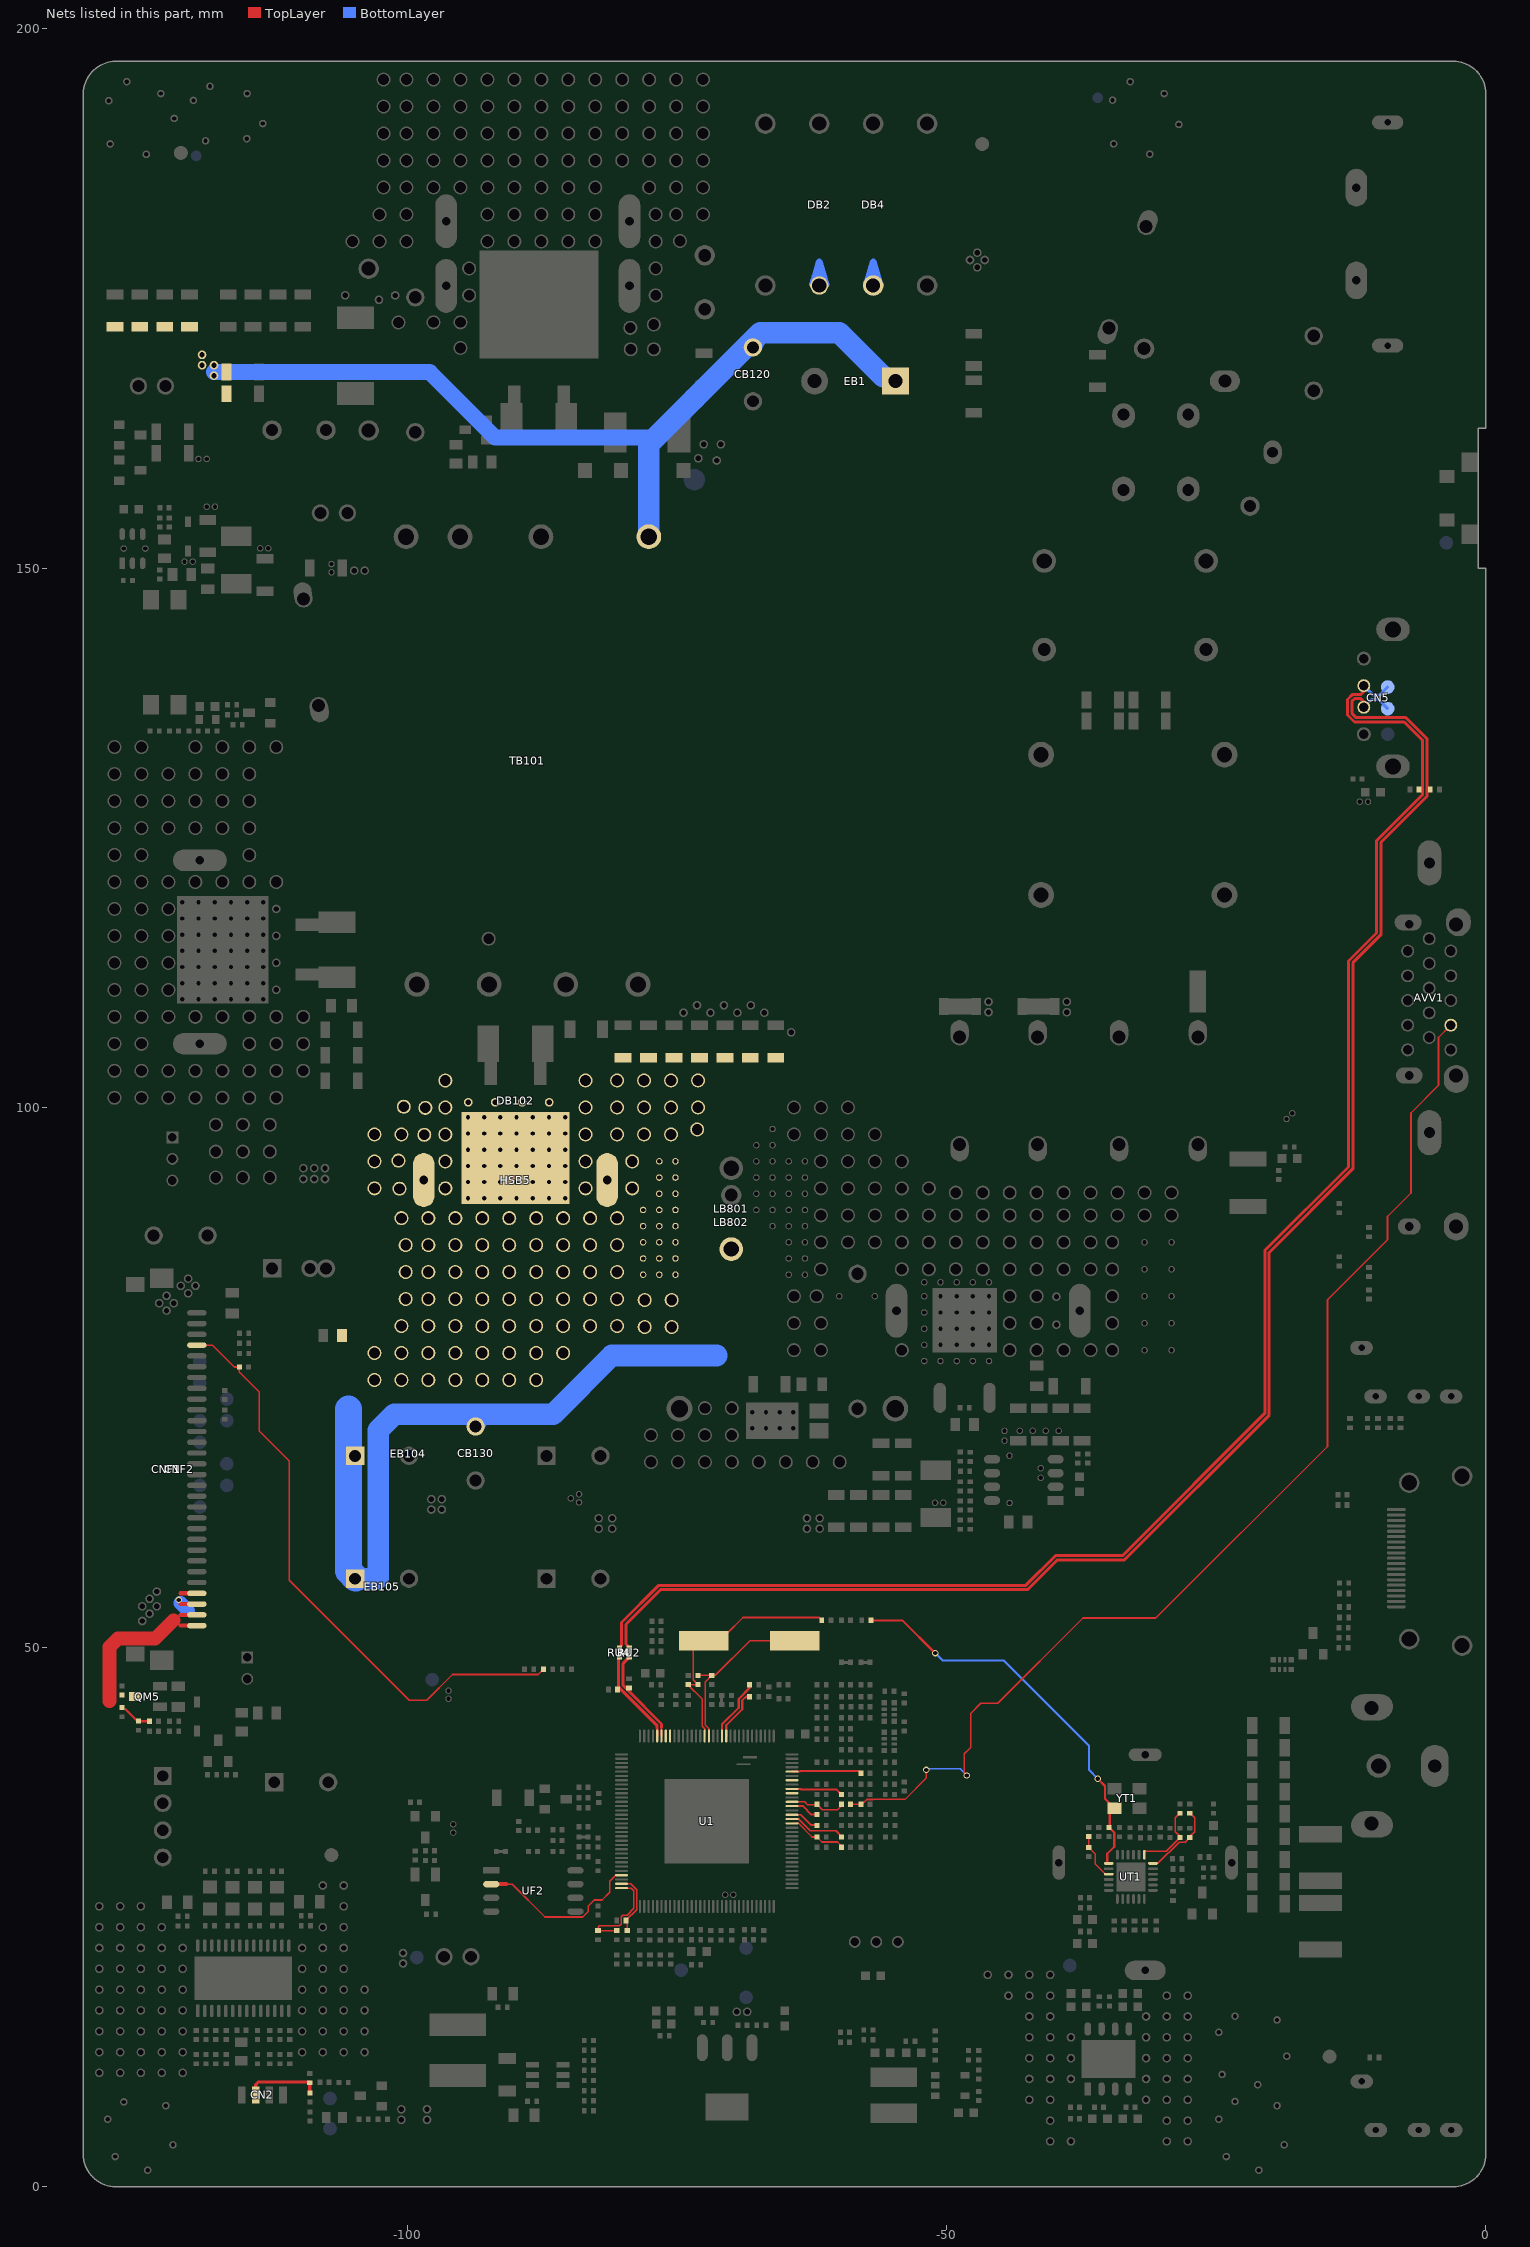
[diagram p0: the nets of this part, all layers, seen from the top]
# Altium PCB MISC84438.PcbDoc (part 13 of 15)
Units mm, origin at the board's own origin, x right, y up, seen from the top; angles counter-clockwise.
Board outline 130 x 197 mm, 2 copper layers (TopLayer, BottomLayer), stack 1.571 mm thick; 574 components, 314 nets, 2636 pads, 811 vias.

## Via types
v1: diameter 0.6, hole 0.4, TopLayer to BottomLayer, tented both sides, 780 vias
v2: diameter 0.7, hole 0.5, TopLayer to BottomLayer, tented both sides, 15 vias
v3: diameter 0.8, hole 0.6, TopLayer to BottomLayer, tented both sides, 12 vias
v4: diameter 0.8, hole 0.5, TopLayer to BottomLayer, tented both sides, 4 vias

## Nets (pads, with @x,y where several pads share a name; then routed paths per layer and width w, separated by ;. In a path a pad name is that pad's centre, name@x,y a point inside that pad or via, vN(x,y) a via of type N, cw(c..) or ccw(c..) an arc to the next point about the centre after c; other vN are vias at no path point) (continued)
SPI_DO: U1.93 UF2.2 | length 15.8
  TopLayer w0.152: -90.805,28.042 -90.246,28.042 -87.203,24.998 -83.721,24.998 -83.185,25.534 -83.185,26.035 -82.652,26.568 -81.928,26.568 -81.204,27.292 -81.204,28.308 -80.642,28.871 U1.93@-80.112,28.871
  TopLayer w0.381: UF2.2@-92.19,28.042 -90.805,28.042
T-IF-AGC: CT1.2 RT2.1 UT1.15 | length 4.4
  TopLayer w0.152: RT2.1@-36.804,32.455 CT1.2@-36.805,31.438 -36.22,30.854 -36.22,29.938 -35.247,28.964 UT1.15@-34.956,28.964
TUNER_SCL: CT8.2 RT6.2 UT1.6 | length 7
  TopLayer w0.127: UT1.6@-30.856,29.964 -30.389,29.964 -28.426,31.928 -27.871,31.928 CT8.2@-27.432,32.366 -27.432,32.472 -26.991,32.912 -26.991,34.174 RT6.2@-27.432,34.614
TUNER_SDA: CT7.2 RT5.2 UT1.7 | length 6.7
  TopLayer w0.127: UT1.7@-31.656,30.764 -31.656,31.019 -31.585,31.09 -29.623,31.09 CT7.2@-28.346,32.366 -28.346,32.472 -28.787,32.912 -28.787,34.174 RT5.2@-28.347,34.614
UART_RX: DH9.K RF11.2 U1.96 | length 9.4
  TopLayer w0.127: RF11.2@-80.543,23.739 DH9.K@-82.296,23.739 -82.296,24.041 -82.169,24.168 -80.313,24.168 -80.146,24.335 -80.146,25.024 -80.016,25.154 -79.606,25.154 -78.969,25.791 -78.969,27.409 -79.231,27.671 U1.96@-80.112,27.671
UART_TX: DH8.K RF10.2 U1.95 | length 6.4
  TopLayer w0.127: U1.95@-80.654,28.071 U1.95@-80.112,28.071 -79.271,28.071 -78.715,27.514 -78.715,25.686 DH8.K@-79.712,24.689 -79.578,24.555 RF10.2@-79.578,23.739
USB0_DM: DU2.K RU2.2 RU2.3 U1.59 | length 9
  TopLayer w0.203: U1.59@-76.412,41.771 -76.412,42.545
  TopLayer w0.279: RU2.2@-79.39,49.079 -79.967,48.502 -79.967,46.453 -79.587,46.073 -76.406,42.892 -76.406,42.551
USB0_DP: DU1.K RU4.2 RU4.3 U1.60 | length 8.8
  TopLayer w0.203: U1.60@-76.812,41.771 -76.812,42.532
  TopLayer w0.279: RU4.2@-80.305,49.079 -80.374,49.01 -80.374,46.285 -80.332,46.243 -76.812,42.723 -76.812,42.532
USB0_M: CN5.2@-11.31,137.13 DU4.K RU2.1 USB0_M.1 | length 152.5
  TopLayer w0.279: RU2.1@-79.39,49.981 -79.705,50.296 -79.705,52.129 -76.5,55.334 -42.477,55.334 -39.708,58.102 -33.485,58.102 -20.079,71.509 -20.079,86.597 -12.332,94.344 -12.332,113.436 -9.728,116.039 -9.728,124.596 -5.448,128.876 -5.448,129.488 -5.448,134.217 -7.401,136.169 -12.014,136.169 -12.421,136.576 -12.421,137.677 -12.171,137.927 -11.587,137.927 -11.31,137.65 CN5.2@-11.31,137.13
  BottomLayer w0.279: CN5.2@-11.31,137.13 -10.594,137.846 -9.942,137.846 USB0_M.1@-9.096,137
USB0_P: CN5.3@-11.31,139.13 DU3.K RU4.1 USB0_P.1 | length 153.1
  TopLayer w0.279: RU4.1@-80.305,49.981 -80.112,50.174 -80.112,52.297 -76.669,55.74 -42.645,55.74 -39.877,58.509 -33.654,58.509 -20.485,71.677 -20.485,86.765 -12.738,94.512 -12.738,113.604 -10.135,116.207 -10.135,124.765 -5.855,129.045 -5.855,129.488 -5.855,134.048 -7.569,135.763 -12.183,135.763 -12.827,136.407 -12.827,137.846 -12.34,138.333 -11.578,138.333 -11.31,138.601 CN5.3@-11.31,139.13
  BottomLayer w0.279: CN5.3@-11.31,139.13 -10.432,138.252 -9.844,138.252 USB0_P.1@-9.096,139
USB1_DM: U1.57
USB1_DP: U1.58
VBL: CB130.2 DB102.2 EB104.1@-104.811,67.742 EB105.1@-104.811,56.35 HSB5.1@-81.448,93.305 HSB5.2 LB801.1@-69.945,86.9 LB802.1 pad.VIA5@-73.1,98 pad.VIA5@-73.023,100.036 pad.VIA5@-73.023,102.536 pad.VIA5@-75.115,84.535 pad.VIA5@-75.115,86.035 pad.VIA5@-75.115,87.535 pad.VIA5@-75.115,89.035 pad.VIA5@-75.115,90.535 pad.VIA5@-75.115,92.035 pad.VIA5@-75.115,93.535 pad.VIA5@-75.115,95.035 pad.VIA5@-75.467,79.68 pad.VIA5@-75.467,82.18 pad.VIA5@-75.523,97.536 pad.VIA5@-75.523,100.036 pad.VIA5@-75.523,102.536 pad.VIA5@-76.615,84.535 pad.VIA5@-76.615,86.035 pad.VIA5@-76.615,87.535 pad.VIA5@-76.615,89.035 pad.VIA5@-76.615,90.535 pad.VIA5@-76.615,92.035 pad.VIA5@-76.615,93.535 pad.VIA5@-76.615,95.035 pad.VIA5@-77.967,79.68 pad.VIA5@-77.967,82.18 pad.VIA5@-78.023,97.536 pad.VIA5@-78.023,100.036 pad.VIA5@-78.023,102.536 pad.VIA5@-78.115,84.535 pad.VIA5@-78.115,86.035 pad.VIA5@-78.115,87.535 pad.VIA5@-78.115,89.035 pad.VIA5@-78.115,90.535 pad.VIA5@-79.123,92.536 pad.VIA5@-79.123,95.036 pad.VIA5@-80.523,79.771 pad.VIA5@-80.523,82.271 pad.VIA5@-80.523,84.771 pad.VIA5@-80.523,87.271 pad.VIA5@-80.523,89.771 pad.VIA5@-80.523,97.536 pad.VIA5@-80.523,100.036 pad.VIA5@-80.523,102.536 pad.VIA5@-83.023,79.771 pad.VIA5@-83.023,82.271 pad.VIA5@-83.023,84.771 pad.VIA5@-83.023,87.271 pad.VIA5@-83.023,89.771 pad.VIA5@-83.448,92.536 pad.VIA5@-83.448,95.036 pad.VIA5@-83.448,97.536 pad.VIA5@-83.448,100.036 pad.VIA5@-83.448,102.536 pad.VIA5@-85.343,91.615 pad.VIA5@-85.343,93.115 pad.VIA5@-85.343,94.615 pad.VIA5@-85.343,96.115 pad.VIA5@-85.343,97.615 pad.VIA5@-85.343,99.115 pad.VIA5@-85.523,77.271 pad.VIA5@-85.523,79.771 pad.VIA5@-85.523,82.271 pad.VIA5@-85.523,84.771 pad.VIA5@-85.523,87.271 pad.VIA5@-85.523,89.771 pad.VIA5@-86.823,100.508 pad.VIA5@-86.843,91.615 pad.VIA5@-86.843,93.115 pad.VIA5@-86.843,94.615 pad.VIA5@-86.843,96.115 pad.VIA5@-86.843,97.615 pad.VIA5@-86.843,99.115 pad.VIA5@-88.023,74.771 pad.VIA5@-88.023,77.271 pad.VIA5@-88.023,79.771 pad.VIA5@-88.023,82.271 pad.VIA5@-88.023,84.771 pad.VIA5@-88.023,87.271 pad.VIA5@-88.023,89.771 pad.VIA5@-88.343,91.615 pad.VIA5@-88.343,93.115 pad.VIA5@-88.343,94.615 pad.VIA5@-88.343,96.115 pad.VIA5@-88.343,97.615 pad.VIA5@-88.343,99.115 pad.VIA5@-89.323,100.508 pad.VIA5@-89.843,91.615 pad.VIA5@-89.843,93.115 pad.VIA5@-89.843,94.615 pad.VIA5@-89.843,96.115 pad.VIA5@-89.843,97.615 pad.VIA5@-89.843,99.115 pad.VIA5@-90.523,74.771 pad.VIA5@-90.523,77.271 pad.VIA5@-90.523,79.771 pad.VIA5@-90.523,82.271 pad.VIA5@-90.523,84.771 pad.VIA5@-90.523,87.271 pad.VIA5@-90.523,89.771 pad.VIA5@-91.343,91.615 pad.VIA5@-91.343,93.115 pad.VIA5@-91.343,94.615 pad.VIA5@-91.343,96.115 pad.VIA5@-91.343,97.615 pad.VIA5@-91.343,99.115 pad.VIA5@-91.823,100.508 pad.VIA5@-92.843,91.615 pad.VIA5@-92.843,93.115 pad.VIA5@-92.843,94.615 pad.VIA5@-92.843,96.115 pad.VIA5@-92.843,97.615 pad.VIA5@-92.843,99.115 pad.VIA5@-93.023,74.771 pad.VIA5@-93.023,77.271 pad.VIA5@-93.023,79.771 pad.VIA5@-93.023,82.271 pad.VIA5@-93.023,84.771 pad.VIA5@-93.023,87.271 pad.VIA5@-93.023,89.771 pad.VIA5@-94.323,100.508 pad.VIA5@-94.343,91.615 pad.VIA5@-94.343,93.115 pad.VIA5@-94.343,94.615 pad.VIA5@-94.343,96.115 pad.VIA5@-94.343,97.615 pad.VIA5@-94.343,99.115 pad.VIA5@-95.523,74.771 pad.VIA5@-95.523,77.271 pad.VIA5@-95.523,79.771 pad.VIA5@-95.523,82.271 pad.VIA5@-95.523,84.771 pad.VIA5@-95.523,87.271 pad.VIA5@-95.523,89.771 pad.VIA5@-96.447,92.536 pad.VIA5@-96.447,95.036 pad.VIA5@-96.447,97.527 pad.VIA5@-96.447,100.027 pad.VIA5@-96.447,102.527 pad.VIA5@-98.3,100 pad.VIA5@-98.4,97.5 pad.VIA5@-98.023,74.771 pad.VIA5@-98.023,77.271 pad.VIA5@-98.023,79.771 pad.VIA5@-98.023,82.271 pad.VIA5@-98.023,84.771 pad.VIA5@-98.023,87.271 pad.VIA5@-98.023,89.771 pad.VIA5@-100.3,100.1 pad.VIA5@-100.7,92.5 pad.VIA5@-100.8,95.1 pad.VIA5@-100.123,82.271 pad.VIA5@-100.123,84.771 pad.VIA5@-100.123,87.271 pad.VIA5@-100.523,74.771 pad.VIA5@-100.523,77.271 pad.VIA5@-100.523,79.771 pad.VIA5@-100.523,89.771 pad.VIA5@-100.523,97.536 pad.VIA5@-103.023,74.771 pad.VIA5@-103.023,77.271 pad.VIA5@-103.023,92.536 pad.VIA5@-103.023,95.036 pad.VIA5@-103.023,97.536 RB124.2 RB125.2 RB126.2 RB127.2 RB140.1 RB162.2 RB163.2 RB164.2 | length 66
  BottomLayer w2: EB105.1@-104.811,56.35 -102.743,56.35 -102.664,56.429 -102.664,70.107 -101.171,71.599 -92.745,71.599 -92.497,71.599 -92.341,71.599 -86.453,71.599 -81.014,77.038 -71.298,77.038
  BottomLayer w2.54: -105.42,72.08 -105.42,68.706 -105.42,68.351 -105.42,67.783 -105.42,57.314 -105.42,57.072 EB105.1@-104.762,56.413
Vbridge: CB120.2 DB2.K DB4.K EB1.1@-54.708,167.359 pad.VIA5@-117.892,167.875 pad.VIA5@-117.892,168.84 pad.VIA5@-118.999,168.834 pad.VIA5@-118.999,169.799 RB117.2 RB118.2 RB150.2 RB151.2 RB152.2 RB156.2 TB101.1 TP-TDT.1 | length 79.7
  BottomLayer w1.5: pad.VIA5@-117.892,168.199 -97.892,168.199 -91.821,162.128 -76.975,162.128
  BottomLayer w2: TB101.1@-77.585,152.942 -77.585,161.518 -76.975,162.128 -68.182,170.92 -67.272,171.831 -66.725,171.831 -66.597,171.831 -66.517,171.831 -59.931,171.831 EB1.1@-55.853,167.752
VCC_PANEL: CF38.1 CM4.1 CM7.2 CNF1.27 CNF1.28 CNF1.29 CNF1.30 CNF2.27 CNF2.28 CNF2.29 CNF2.30 QM5.D RM6.1 VCC_PANEL.1 | length 21.7
  TopLayer w0.203: -126.086,44.247 -124.999,43.16 RM6.1@-124.892,43.16 -124.873,43.142 CM7.2@-123.882,43.142
  TopLayer w0.381: -121.004,52 CNF2.30@-119.486,52 ; -121.004,53 CNF2.29@-119.486,53 ; -121.004,54 CNF2.28@-119.486,54 ; -121.004,55 CNF2.27@-119.486,55
  TopLayer w1.27: -127.584,44.983 -127.584,50.013 -126.785,50.812 -123.33,50.812 -121.641,52.502
  BottomLayer w1.27: -120.999,54.091 VCC_PANEL.1@-120.326,53.418
  other v1: -121.156,54.379
VCOM0: CF26.1 U1.28 | length 6.5
  TopLayer w0.198: U1.28@-64.312,38.471 -63.611,38.471 -63.546,38.536 -58.163,38.536 CF26.1@-57.931,38.303
VGA_BIN: CV7.1 U1.17 | length 5.3
  TopLayer w0.18: -63.692,34.071 -62.608,32.987 -60.234,32.987 CV7.1@-59.734,32.487
  TopLayer w0.198: U1.17@-64.312,34.071 -63.692,34.071 ; CV7.1@-59.734,32.41 CV7.1@-59.734,32.487
VGA_GIN: CV3.1 U1.18 | length 2.7
  TopLayer w0.18: U1.18@-64.312,34.471 -63.503,34.471 -62.56,33.528 CV3.1@-62.02,33.528
VGA_HS: CV9.2 RV12.2 U1.16 | length 5.5
  TopLayer w0.152: U1.16@-64.312,33.671 -63.719,33.671 -62.459,32.41 CV9.2@-61.995,32.41 -61.533,31.948 -60.092,31.948 RV12.2@-59.715,31.572
VGA_RIN: CV1.1 U1.20 | length 2.6
  TopLayer w0.18: U1.20@-64.312,35.271 -63.287,35.271 -62.509,34.493 CV1.1@-61.995,34.493
VGA_VS: CV10.2 RV10.2 U1.21 | length 5.2
  TopLayer w0.152: U1.21@-64.312,35.671 -63.144,35.671 -62.881,35.407 CV10.2@-61.995,35.407 ; CV10.2@-61.995,35.433 -61.508,34.946 -60.1,34.946 -59.734,35.313 RV10.2@-59.734,35.433
VIFM: CT23.2 U1.45 | length 5.8
  TopLayer w0.203: U1.45@-70.812,41.771 -70.812,42.832 -69.253,44.391 -69.253,45.21 -68.25,46.213 CT23.2@-68.25,46.507
VIFP: CT20.2 U1.44 | length 4.7
  TopLayer w0.203: U1.44@-70.412,41.771 -70.412,42.765 -68.923,44.254 -68.923,45.073 -68.581,45.415 CT20.2@-68.25,45.415
Vs: CK4.1 CN2.2 RK13.2 | length 7
  TopLayer w0.305: CN2.2@-114.035,8.502 -114.035,9.434 -113.767,9.703 CK4.1@-109.004,9.703 ; RK13.2@-109.004,8.705 CK4.1@-109.004,9.633
VS_VGA: AVV1.14 RV10.1 RV14.1 | length 106
  TopLayer w0.152: RV10.1@-58.884,35.433 RV14.1@-57.931,35.433 ; RV14.1@-57.931,35.44 RV14.1@-57.931,35.433 ; v1(-51.862,38.625) -51.862,37.87 -53.838,35.894 -56.771,35.894 -56.779,35.886 -57.39,35.886 -57.843,35.433 RV14.1@-57.931,35.433 ; v1(-48.112,38.111) -48.336,38.334 -48.336,40.119 -47.758,40.697 -47.758,43.851 -46.816,44.793 -45.246,44.793 -37.334,52.705 -30.587,52.705 -14.681,68.611 -14.681,80.772 -14.681,82.21 -9.119,87.772 -9.119,89.924 -6.934,92.109 -6.934,99.526 -4.383,102.078 -4.383,106.525 AVV1.14@-3.247,107.66
  BottomLayer w0.152: v1(-51.862,38.625) -51.765,38.722 -48.714,38.722 -48.112,38.12 v1(-48.112,38.111)
WP//SCL: CNF1.4 CNF2.4 RF22.2 RF25.2 | length 55.8
  TopLayer w0.152: CNF2.4@-119.486,78 -118.037,78 -116.009,75.972 RF22.2@-115.543,75.972 -115.543,75.506 -113.695,73.658 -113.695,70.047 -110.915,67.267 -110.915,56.2 -99.8,45.085 -98.168,45.085 -95.78,47.473 -87.826,47.473 RF25.2@-87.344,47.955
XTAL_O: CF40.1 CT14.2 UT1.13 YT1.1 | length 37.8
  TopLayer w0.203: CF40.1@-57.004,52.489 -54.089,52.489 -51.063,49.463 v1(-51.038,49.463) ; v1(-35.97,37.822) -35.294,37.146 -35.294,35.958 YT1.1@-34.415,35.079 ; UT1.13@-35.244,29.964 -35.1,30.109 ; UT1.13@-34.956,29.964 -35.1,30.109 ; YT1.1@-34.868,35.219 -34.868,33.361 CT14.2@-34.925,33.305 -34.446,32.826 -34.446,31.505 -35.1,30.851 -35.1,30.109
  BottomLayer w0.203: v1(-51.038,49.463) -50.343,48.768 -44.68,48.768 -36.788,40.876 -36.788,38.64 v1(-35.97,37.822)
XTALI: CF4.2 RF1.1 U1.48 YF1.1 | length 16.3
  TopLayer w0.152: RF1.1@-73.025,47.389 CF4.2@-71.755,47.389 ; U1.48@-72.012,41.771 -72.012,42.434 -72.365,42.786 -72.365,46.78 CF4.2@-71.755,47.389 ; YF1.1@-64.068,50.594 -68.215,50.594 -71.419,47.389 CF4.2@-71.755,47.389
XTALO: CF1.2 RF1.2 RF24.2 U1.49 YF1.2 | length 20.8
  TopLayer w0.152: RF1.2@-73.034,46.53 -73.965,46.53 -72.644,45.209 -72.644,42.671 -72.412,42.439 U1.49@-72.412,41.771 ; RF1.2@-73.025,46.539 -73.478,46.993 -73.478,49.988 -72.872,50.594 YF1.2@-72.483,50.594 ; YF1.2@-70.358,51.257 -68.859,52.756 -61.817,52.756 RF24.2@-61.55,52.489
YPBPR_PB: U1.23
YPBPR_PR: U1.26
YPBPR_Y: CI1.1 U1.24 | length 4.8
  TopLayer w0.198: U1.24@-64.312,36.871 -63.525,36.871
  TopLayer w0.203: -63.525,36.871 -63.48,36.826 -60.213,36.826 CI1.1@-59.734,36.347
pads on no net: "Conformal Coating.0" AI_V.0 AI_V.1 AI_V.2 AVH1.4@-2.9,50.55 AVH1.4@-2.9,65.45 AVH1.4@-7.2,50.75 AVH1.4@-7.2,65.25 AVI1.0 AVI2.0 AVO1.0 AVO2.0 AVO2.4 AVV1.0 AVV1.4 AVV1.9 AVV1.11 AVV1.30 AVV1.31 AVV1.32 AVV1.33 AVV1.34 AVV1.35 AVV1.36 AVV1.37 AVV1.38 AVV1.39 AVV1.40 AVV1.41 AVV1.42 AVV1.43 AVV1.44 BB101.35 BB101.36 BB801.35 BB801.36 CB114.1@-107.507,162.814 CB114.1@-112.507,162.814 CB116.0 CB120.41 CB120.42 CB130.41 CB130.42 CB808.41 CB808.42 CN5.0 CN5.1@-11.31,137.13 CN5.2@-11.31,139.13 CN5.3@-11.31,141.63 CN9.0 CNA1.0 CNA2.0 CNA3.0 CNB1.0 CNB1.1@-9.1,170.65 CNB1.1@-9.1,191.35 CNB1.1@-12,176.7 CNB1.1@-12,185.3 CNB1.3 CNB1.4 CNB2.0 CNB832.0 CNB833.0 CXB1.77 CXB1.78 CXB2.3 CXB2.4 CYB1.61 CYB2.61 CYB3.61 CYB4.61 CYB5.61 CYB6.61 DB1.15 DB1.16 DB2.15 DB2.16 DB3.15 DB3.16 DB4.15 DB4.16 DB106.15 DB106.16 DB801.0 DB801.1 EA1.0 EA1.1@-107.304,37.486 EA1.1@-112.304,37.486 EB1.1@-54.708,167.359 EB1.1@-62.208,167.359 EB101.0 EB101.1@-107.5,85.114 EB101.1@-112.5,85.114 EB102.1@-109,85.114 EB102.1@-112.5,85.114 EB104.0 EB104.1@-99.811,67.742 EB104.1@-104.811,67.742 EB105.0 EB105.1@-99.811,56.35 EB105.1@-104.811,56.35 EB106.0 EB107.0 EB801.0 EB801.1@-82.073,67.742 EB801.1@-87.073,67.742 EB802.0 EB802.1@-82.073,56.35 EB802.1@-87.073,56.35 ED2.0 ED2.5 ED2.6 FB1.4 FB1.5 H1.0 H1.1@-19.225,5.725 H1.1@-20.34,7.339 H1.1@-22.232,7.859 H1.1@-24.015,7.041 H1.1@-24.856,5.268 H2.0 H2.1@-19.225,13.725 H2.1@-19.408,11.772 H2.1@-20.34,15.339 H2.1@-20.804,10.393 H2.1@-22.76,10.234 H2.1@-22.232,15.859 H2.1@-24.015,15.041 H2.1@-24.36,11.37 H2.1@-24.856,13.268 H3.0 H3.1@-122.225,5.725 H3.1@-123.34,7.339 H3.1@-125.232,7.859 H3.1@-127.015,7.041 H3.1@-127.856,5.268 H4.0 H4.1@-29.225,192.725 H4.1@-29.408,190.772 H4.1@-30.804,189.393 H4.1@-32.76,189.234 H4.1@-34.36,190.37 H4.1@-34.856,192.268 H5.0 H5.1@-122.225,192.725 H5.1@-122.408,190.772 H5.1@-123.804,189.393 H5.1@-125.76,189.234 H5.1@-127.36,190.37 H5.1@-127.856,192.268 H6.0 H6.1@-114.225,192.725 H6.1@-114.408,190.772 H6.1@-115.804,189.393 H6.1@-117.76,189.234 H6.1@-119.36,190.37 H6.1@-119.856,192.268 HSB1.1@-79.374,176.188 HSB1.1@-96.374,176.188 HSB2.1@-79.374,182.188 HSB2.1@-96.374,182.188 HSB3.1@-119.2,105.938 HSB3.1@-119.2,122.938 HSB4.1@-37.626,81.193 HSB4.1@-54.626,81.193 HSB5.1@-81.448,93.305 HSB5.1@-98.448,93.305 JP1.1@-27.582,157.263 JP1.1@-27.582,164.263 JP2.1@-33.582,157.263 JP2.1@-33.582,164.263 LB801.1@-69.945,86.9 LB801.1@-69.946,94.4 LB802.3 LB802.4 LCB1.5 LCB1.6 LCB1.7 LCB1.8 LCB2.0 M1.0 M2.0 M3.0 M4.0 Manufacture_Info.0 MOVB1.2@-24.182,167.366 MOVB1.2@-31.682,170.366 NTCB1.2@-21.862,155.768 NTCB1.3 PT1.0 RFT1.0 RFT2.0 S/N1.0 S/N2.0 SK1. TB101.0 U1.9@-69.912,31.571 U1.9@-69.912,33.871 U1.9@-69.912,36.171 U1.9@-72.212,31.571 U1.9@-72.212,33.871 U1.9@-72.212,36.171 U1.9@-74.512,31.571 U1.9@-74.512,33.871 U1.9@-74.512,36.171 UA1.13 UA1.EPAD@-112.748,18.64 UA1.EPAD@-112.748,19.99 UA1.EPAD@-114.366,18.64 UA1.EPAD@-114.366,19.99 UA1.EPAD@-115.984,18.64 UA1.EPAD@-115.984,19.99 UA1.EPAD@-117.602,18.64 UA1.EPAD@-117.602,19.99 UT1.14 UT1.21 XXXXXX.0 XXXXXXXXXXXXXXX.0 用于U1上方.0
copper on no net: | length 86.4
  TopLayer w0.127: 186.36,29.431 186.36,31.431 ; 172.367,29.431 190.96,29.431 190.96,31.431 172.367,31.431 172.367,29.431
  BottomLayer w0.127: 186.36,23.897 186.36,25.897 ; 172.367,23.897 172.367,25.897 190.96,25.897 190.96,23.897 172.367,23.897

## Polygon pours and split planes (outlines as drawn)
GND on BottomLayer "GND" (solid, remove dead copper, pour order 30): -111.9,75.6 -111.9,77.2 -108.1,81 -105.8,83.3 -105.8,84.1 -105.8,85.1 -106.1,85.4 -106.4,85.7 -107.8,85.7 -111.1,85.7 -111.2,85.6 -111.345,85.455 -111.345,84.709 -111.345,84.055 -111.6,83.8 -112.8,82.6 -112.8,80.8 -112.8,76.6 -112.1,75.9
GND on BottomLayer "12" (solid, remove dead copper, pour order 21): -99.898,68.605 -90.17,68.605 -89.154,67.589 -89.154,56.083 -90.729,54.508 -99.238,54.508 -100.609,55.88 -100.609,67.818 -99.822,68.605
GND on BottomLayer "12" (solid, remove dead copper, pour order 26): -116.891,197.079 -115.189,197.079 cw(c-115.189,194.158) -112.268,194.158 -112.268,193.548 -112.268,189.789 cw(c-114.808,189.789) -114.808,187.249 -116.891,187.249 -126.771,187.249 cw(c-126.771,190.525) -130.048,190.525 -130.048,191.948 -130.048,194.46 cw(c-127.508,194.46) -127.508,197 -126.517,197
GND on BottomLayer "12" (solid, remove dead copper, pour order 25): -32.004,196.952 -29.896,196.952 cw(c-29.896,194.056) -27,194.056 -27,190.094 cw(c-29.82,190.094) -29.82,187.274 -32.004,187.274 -33.884,187.274 cw(c-33.884,190.246) -36.855,190.246 -36.855,192.227 -36.855,194.031 cw(c-33.934,194.031) -33.934,196.952 -32.106,196.952
SGND on BottomLayer "12" (solid, remove dead copper, pour order 22): -123.383,166.335 -124.859,164.859 -124.859,156.573 -127.94,153.492 -127.94,150.165 -127.279,149.504 -121.488,149.504 -121.183,149.809 -121.183,150.952 -119.177,152.959 -119.177,162.128
GND on BottomLayer "5" (solid, remove dead copper, pour order 29): -115.545,78.651 -119.407,78.651 -123.152,74.907 -123.152,72.39 -123.152,63.627 -119.736,60.211 -113.716,60.211 -113.386,60.541 -113.525,60.681 -113.525,77.572 -114.579,78.626 -114.973,78.626
RFGND on BottomLayer "12" (solid, remove dead copper, pour order 38): 0,45.949 -14.823,45.949 -14.834,45.938 -19.192,41.58 -19.192,25.324 -18.961,25.093 -0.155,25.093 0,25.248
GND on BottomLayer "12" (solid, remove dead copper, pour order 37): -0.703,150.703 0,150 0,1.816 -1.816,0 -128.143,0 -130.061,1.918 -130.061,83.185 -128.537,84.709 -110.515,84.709 -110.414,84.607 -111.3,83.721 -111.3,55.141 -107.112,50.952 -86.081,50.952 -78.664,58.369 -44.238,58.369 -41.063,61.544 -39.078,61.544 -26.416,74.206 -26.416,95.265 -24.297,97.384 -21.312,97.384 -14.173,104.523 -14.173,115.427 -11.57,118.03 -11.57,125.438 -13.856,127.724 -13.856,142.567 -6.413,150.009 -6.413,157.201 -3.035,160.579 -0.703,160.579
D_QB101 on TopLayer "12" (solid, remove dead copper, pour order 28): -75.501,169.47 -105.868,169.47 -106.451,170.053 -106.451,180.924 -102.819,184.556 -102.819,196.139 -102.502,196.456 -71.349,196.456 -70.866,195.974 -70.866,177.927 -71.552,177.241 -73.711,177.241 -75.501,175.451
D_QB801 on TopLayer "12" (solid, remove dead copper, pour order 27): -29.7,93.8 -27.771,91.871 -27.771,76.568 -28.596,75.743 -59.245,75.743 -60.071,76.568 -66.845,76.568 -67.457,77.18 -67.457,88.514 -68.707,89.764 -70.16,89.764 -70.775,90.378 -70.775,94.894 -63.828,101.841 -59.941,101.841 -51.9,93.8
GND on TopLayer "12" (solid, remove dead copper, pour order 35): -0.703,150.703 0,150 0,1.816 -1.816,0 -128.143,0 -130.061,1.918 -130.061,83.185 -128.537,84.709 -112.865,84.709 -112.865,72.136 -108.852,68.123 -108.852,56.841 -101.689,49.678 -84.613,49.678 -83.81,50.482 -83.81,52.676 -78.117,58.369 -44.238,58.369 -41.063,61.544 -39.078,61.544 -26.416,74.206 -26.416,93.025 -25.654,93.787 -24.092,93.787 -14.173,103.706 -14.173,114.198 -11.57,116.802 -11.57,125.438 -13.856,127.724 -13.856,142.567 -5.447,150.976 -5.447,158.167 -3.035,160.579 -0.703,160.579
RFGND on TopLayer "12" (solid, remove dead copper, pour order 36): 0,45.949 -14.823,45.949 -14.834,45.938 -19.192,41.58 -19.192,25.324 -18.961,25.093 -0.155,25.093 0,25.248
GND on TopLayer "5" (solid, remove dead copper, pour order 34): -80.556,44.869 -81.216,45.529 -81.216,52.755 -77.406,56.566 -42.888,56.566 -40.373,59.08 -34.112,59.08 -21.26,71.933 -21.26,86.931 -13.538,94.653 -13.538,113.767 -10.706,116.599 -10.706,125.451 -6.769,129.388 -6.769,133.172 -8.039,134.442 -10.274,134.442 -10.274,137.795 -9.792,138.278 -7.429,138.278 -3.264,134.112 -3.264,129.007 -3.861,129.007 -8.433,124.435 -8.433,115.667 -11.76,112.34 -11.76,93.701 -19.507,85.954 -19.507,70.79 -32.982,57.315 -39.172,57.315 -42.181,54.305 -75.959,54.305 -78.383,51.881 -78.383,43.966 -78.651,44.234 -80.505,44.234
GND on TopLayer "12" (solid, remove dead copper, pour order 20): -102.286,68.58 -102.286,55.397 -102.286,51.105 -90.83,51.105 -89.103,52.832 -89.103,57.937 -88.341,58.699 -84.099,58.699 -82.779,58.699 -80.62,60.858 -81.991,62.23 -85.217,62.23 -88.951,65.964 -88.951,67.666 -89.865,68.58 -102.133,68.58 -102.184,68.529
GND on TopLayer "12" (solid, remove dead copper, pour order 23): -116.891,197.079 -115.189,197.079 cw(c-115.189,194.158) -112.268,194.158 -112.268,193.548 -112.268,189.789 cw(c-114.808,189.789) -114.808,187.249 -116.891,187.249 -126.771,187.249 cw(c-126.771,190.525) -130.048,190.525 -130.048,191.948 -130.048,194.46 cw(c-127.508,194.46) -127.508,197 -126.517,197
GND on TopLayer "12" (solid, remove dead copper, pour order 24): -32.004,196.952 -29.896,196.952 cw(c-29.896,194.056) -27,194.056 -27,190.094 cw(c-29.82,190.094) -29.82,187.274 -32.004,187.274 -33.884,187.274 cw(c-33.884,190.246) -36.855,190.246 -36.855,192.227 -36.855,194.031 cw(c-33.934,194.031) -33.934,196.952 -32.106,196.952
GND on TopLayer "6.2" (solid, remove dead copper, pour order 33): -6.756,115.646 -7.899,115.646 -8.421,115.125 -10.884,112.662 -10.884,111.188 -10.884,93.828 -11.697,93.015 -14.826,89.885 -14.826,89.802 -18.631,85.998 -18.631,82.906 -18.631,70.955 -21.171,68.415 -32.931,56.655 -36.17,56.655 -38.964,56.655 -39.599,56.02 -45.587,50.032 -47.574,50.032 -48.228,50.032 -50.495,47.765 -52.248,46.012 -52.248,40.665 -52.248,37.338 -53.454,36.131 -54.077,35.509 -56.388,35.509 -56.889,35.509 -57.905,34.493 -57.905,31.743 -57.315,31.153 -55.184,31.153 -53.176,33.161 -49.2,37.138 -49.2,39.674 -49.2,45.6 -48.314,46.485 -47.683,47.117 -46.101,47.117 -45.136,47.117 -43.536,48.717 -37.846,54.407 -33.795,54.407 -31.953,54.407 -31.521,54.839 -16.345,70.015 -16.345,77.14 -16.345,85.026 -14.618,86.754 -14.029,87.343 -12.738,87.343 -12.738,87.452 -12.052,88.138 -10.643,89.548 -10.643,90.555 -10.643,90.614 -10.008,91.249 -8.458,92.799 -8.458,95.834 -8.458,108.077 -8.052,108.483 -8.001,108.534 -6.642,108.534 -6.096,109.08 -6.134,109.118 -6.134,115.379 -6.401,115.646 -6.756,115.646
GND on TopLayer "5" (solid, remove dead copper, pour order 31): -6.714,62.772 -7.149,63.208 -9.856,63.208 -10.592,62.471 -16.015,62.471 -29.032,49.454 -36.119,49.454 -54.597,30.975 -62.611,30.975 -63.573,30.013 -63.573,27.834 -63.823,27.584 -64.897,27.584 -64.897,27.429 -65.862,26.464 -65.862,25.66 -66.542,24.981 -66.802,24.981 -66.802,24.765 -65.38,23.343 -61.163,23.343 -59.201,25.305 -51.949,25.305 -33.655,43.599 -26.721,43.599 -13.386,56.934 -9.56,56.934 -9.244,57.25 -9.244,62.544 -9.025,62.763 -6.722,62.763
GND on TopLayer "5" (solid, remove dead copper, pour order 32): -118.389,77.292 -120.923,77.292 -121.186,77.029 -121.186,62.029 -120.957,61.8 -118.364,61.8 -118.364,53.411 -102.443,37.49 -81.583,37.49 -81,38.073 -81,39.752 -80.682,40.071 -79.64,40.071 -78.412,41.298 -78.412,42.18 -78.523,42.291 -78.086,42.728 -76.119,42.728 -76.035,42.812 -76.035,43.745 -78.912,46.622 -80.569,46.622 -82.448,44.742 -99.475,44.742 -111.1,56.367 -111.1,67.234 -113.894,70.028 -113.894,73.812 -116.23,76.149

## Keep-outs
KeepOutLayer:
  rectangle: 172.367,14.26 175.674,16.26
  pour cut-out: -20.814,24.258 -20.027,23.471 ccw(c-19.355,24.143) -19.355,23.192 -0.343,23.192 ccw(c-0.343,24.143) 0.607,24.143 ccw(c-0.343,24.143) -0.343,25.093 -18.961,25.093 -19.192,25.324 -19.192,41.58 -14.834,45.938 0,45.938 ccw(c0,46.888) 0.95,46.888 ccw(c0,46.888) 0,47.839 -15.227,47.839 ccw(c-15.227,46.888) -15.899,47.56 -20.814,42.646 ccw(c-20.142,41.974) -21.093,41.974 -21.093,24.93 ccw(c-20.142,24.93)
  lines w0.127: 186.36,14.26 186.36,16.26 ; -130,3 ccw(c-127,3) -127,0 -3,0 ccw(c-3,3) 0,3 0,150 -0.703,150 -0.703,163 ; -130,3 cw(c-133,3) -133,0 -257,0 cw(c-257,3) -260,3 -260,34 -259.297,34 -259.297,47 -260,47 -260,194 cw(c-257,194) -257,197 -133,197 cw(c-133,194) -130,194 ; -130,3 -130,194 ; -130,3 -130,194 ; -130,194 cw(c-127,194) -127,197 -3,197 ; -3,197 cw(c-3,194) 0,194 ; -3,197 cw(c-3,194) 0,194 ; -0.703,163 0,163 ; -0.703,163 0,163 ; -0.703,163 0,163 ; -0.703,163 0,163 ; 0,163 -0.703,163 0,163 ; 0,163 0,194 ; -96.304,126.619 ccw(c-95.034,126.619) -95.034,125.349 -75.26,125.349 ccw(c-75.26,126.619) -73.99,126.619 -73.99,145.796 ccw(c-75.26,145.796) -75.26,147.066 -95.034,147.066 ccw(c-95.034,145.796) -96.304,145.796 -96.304,128.295 -96.304,126.619 ; 172.367,14.26 172.367,16.26 190.96,16.26 190.96,14.26 172.367,14.26
  lines w1.2: -51.841,180.264 -48.692,177.114
  text "KeepOutLayer" at 176.248,14.792 h1.52
  text ".GKO" at 186.962,14.718 h1.52